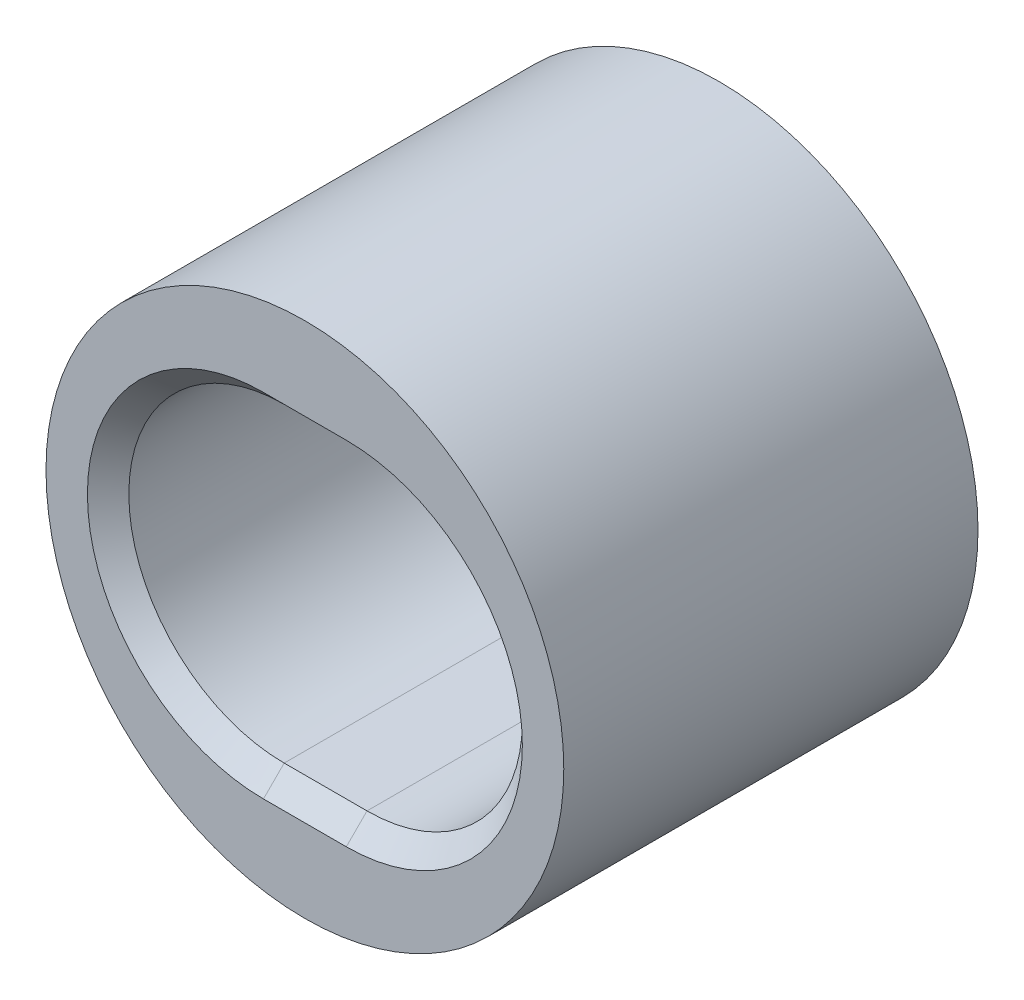
from build123d import *

# Parameters (mm, degrees)
SKETCH1_R           = 12.5
BOSS_EXTRUDE1_DEPTH = 20
CHAMFER1_SIZE       = 1


with BuildPart() as part:
    # Sketch1 → Boss-Extrude1 (new body)
    with BuildSketch(Plane.XY):
        Circle(SKETCH1_R)
        with BuildLine():
            Line((-2, 7.5), (2, 7.5))
            ThreePointArc((2, 7.5), (9.5, 0), (2, -7.5))
            Line((2, -7.5), (-2, -7.5))
            ThreePointArc((-2, -7.5), (-9.5, 0), (-2, 7.5))
        make_face(mode=Mode.SUBTRACT)
    extrude(amount=BOSS_EXTRUDE1_DEPTH)

    # Chamfer1
    chamfer1_edges = [part.edges().sort_by_distance(p)[0] for p in [
        (0, 7.5, 20),
        (-9.5, 0, 20),
        (0, -7.5, 20),
        (9.5, 0, 20),
    ]]
    chamfer(chamfer1_edges, length=CHAMFER1_SIZE)


solid = part.part
